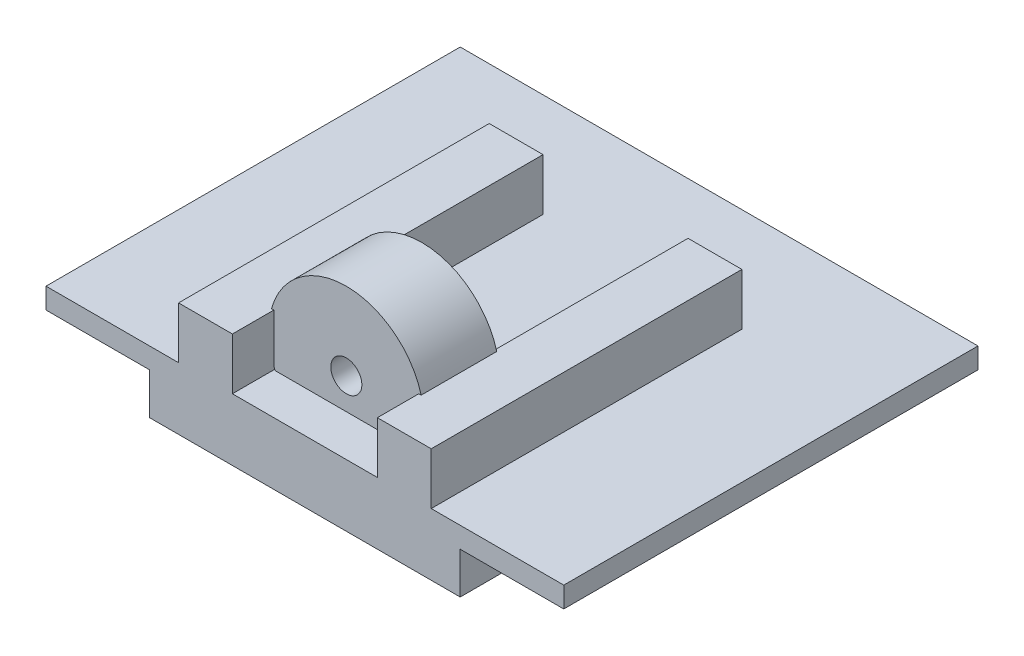
from build123d import *

# Parameters (mm, degrees)
SKETCH1_W           = 500
SKETCH1_H           = 400
BOSS_EXTRUDE1_DEPTH = 20
SKETCH2_W           = 52
SKETCH2_H           = 300
BOSS_EXTRUDE2_DEPTH = 50
SKETCH3_W           = 300
SKETCH3_H           = 400
BOSS_EXTRUDE3_DEPTH = 40
SKETCH6_R           = 75
BOSS_EXTRUDE5_DEPTH = 73
SKETCH7_R           = 15
CUT_EXTRUDE2_DEPTH  = 456.768581629


with BuildPart() as part:
    # Sketch1 → Boss-Extrude1 (new body)
    with BuildSketch(Plane(origin=(0, 0, 0), x_dir=(1, 0, 0), z_dir=(0, 1, 0))):
        Rectangle(SKETCH1_W, SKETCH1_H)
    extrude(amount=BOSS_EXTRUDE1_DEPTH)

    # Sketch2 → Boss-Extrude2 (add)
    with BuildSketch(Plane(origin=(0, 20, 0), x_dir=(1, 0, 0), z_dir=(0, 1, 0))):
        with Locations((-96, -50)):
            Rectangle(SKETCH2_W, SKETCH2_H)
        with Locations((96, -50)):
            Rectangle(SKETCH2_W, SKETCH2_H)
    extrude(amount=BOSS_EXTRUDE2_DEPTH)

    # Sketch3 → Boss-Extrude3 (add)
    with BuildSketch(Plane.XZ):
        Rectangle(SKETCH3_W, SKETCH3_H)
    extrude(amount=BOSS_EXTRUDE3_DEPTH)

    # Sketch6 → Boss-Extrude5 (add)
    with BuildSketch(Plane.XY.offset(160)):
        with Locations((0, 50)):
            Circle(SKETCH6_R)
    extrude(amount=-BOSS_EXTRUDE5_DEPTH)

    # Sketch7 → Cut-Extrude2 (cut, through all)
    with BuildSketch(Plane.XY.offset(160)):
        with Locations((0, 50)):
            Circle(SKETCH7_R)
    extrude(amount=-CUT_EXTRUDE2_DEPTH, mode=Mode.SUBTRACT)


solid = part.part
